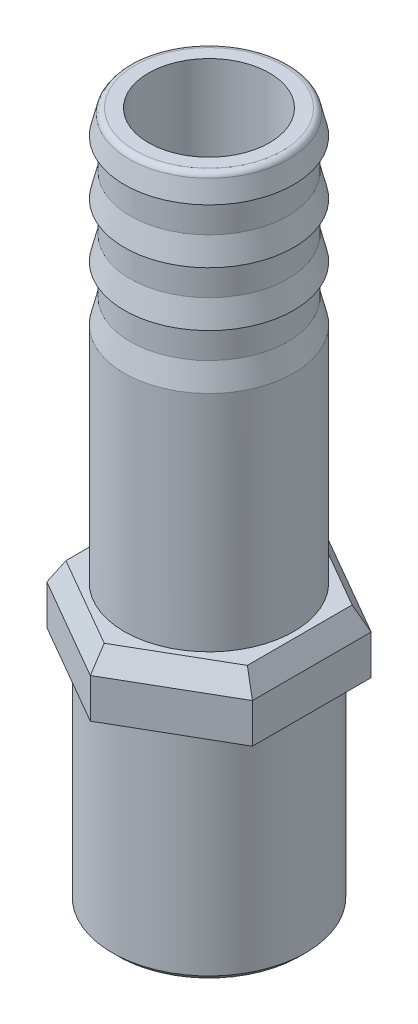
SolidWorks part; units mm, degrees
material "AISI 304"
ref_plane "Front Plane" through (0, 0, 0) normal (0, 0, 1) x (1, 0, 0)
ref_plane "Top Plane" through (0, 0, 0) normal (0, 1, 0) x (1, 0, 0)
ref_plane "Right Plane" through (0, 0, 0) normal (1, 0, 0) x (0, 0, -1)
sketch "Sketch2" plane through (0, 0, 0) normal (0, 1, 0) x (1, 0, 0)
  circle A0 centre (0, 0) radius 7
  dimension "D1" = 14
extrude "Boss-Extrude1" add sketch "Sketch2" along normal blind 34
sketch "Sketch3" plane through (0, 0, 0) normal (0, 0, 1) x (1, 0, 0)
  line L0 (0, 0) -> (0, 64.2773) construction
  line L1 (6.5, 34) -> (7, 32)
  line L2 (7, 32) -> (6.5, 32)
  line L7 (7, 34) -> (-7, 34) construction
  line L8 (7, 0) -> (7, 34) construction
  line L9 (6.5, 34) -> (7, 34)
  line L10 (7, 34) -> (7, 18.5)
  line L11 (-7, 17) -> (14.6266, 17) construction
  line L12 (-7, 34) -> (-7, 0) construction
  line L13 (6.5, 32) -> (6.5, 29.5)
  line L14 (6.5, 29.5) -> (7, 27.5)
  line L15 (7, 27.5) -> (6.5, 27.5)
  line L16 (6.5, 27.5) -> (6.5, 25)
  line L17 (6.5, 25) -> (7, 23)
  line L18 (7, 23) -> (6.5, 23)
  line L20 (6.5, 23) -> (6.5, 20.5)
  line L21 (6.5, 20.5) -> (7, 18.5)
  dimension "D1" = 6.5
  dimension "D2" = 2
  dimension "D3" = 4.5
  dimension "D4" = 0.5
revolve "Cut-Revolve1" cut sketch "Sketch3" angle 360 about L0
sketch "Sketch5" plane through (0, 0, 0) normal (0, -1, 0) x (1, 0, 0)
  line L1 (8.5, -4.9075) -> (8.5, 4.9075)
  line L2 (8.5, 4.9075) -> (0, 9.815)
  line L3 (0, 9.815) -> (-8.5, 4.9075)
  line L4 (-8.5, 4.9075) -> (-8.5, -4.9075)
  line L5 (-8.5, -4.9075) -> (0, -9.815)
  line L6 (0, -9.815) -> (8.5, -4.9075)
  circle A0 centre (0, 0) radius 8.5 construction
  dimension "D1" = 17
extrude "Boss-Extrude2" add sketch "Sketch5" along normal blind 5
sketch "Sketch6" plane through (0, -5, 0) normal (0, -1, 0) x (1, 0, 0)
  circle A0 centre (0, 0) radius 8
  dimension "D1" = 16
extrude "Boss-Extrude3" add sketch "Sketch6" along normal blind 18
sketch "Sketch4" plane through (0, 34, 0) normal (0, 1, 0) x (1, 0, 0)
  circle A0 centre (0, 0) radius 5
  dimension "D1" = 10
extrude "Cut-Extrude1" cut sketch "Sketch4" against normal through all
chamfer "Chamfer1" distance 1 angle 60 6 edges at (-4.25, 0, 7.3612) (-8.5, 0, 0) (-4.25, 0, -7.3612) (4.25, 0, -7.3612) (8.5, 0, 0) (4.25, 0, 7.3612)
chamfer "Chamfer3" distance 0.5 angle 45 1 edges at (0, -23, -8)
fillet "Fillet1" radius 0.5 1 edges at (0, 34, -6.5)
